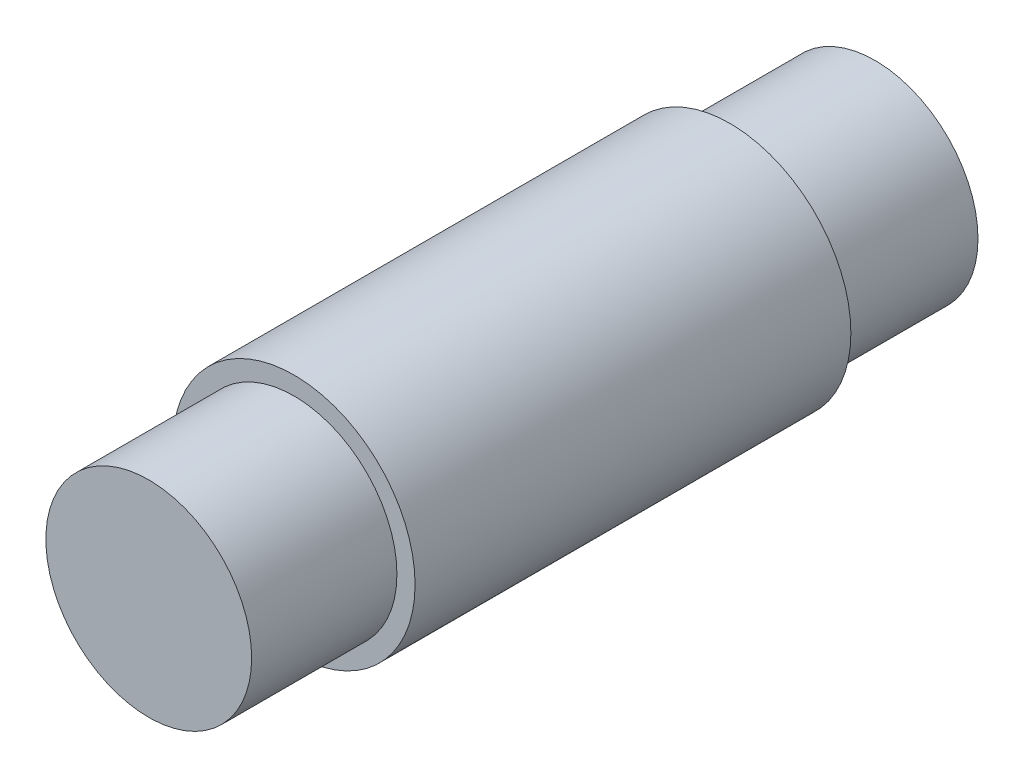
from build123d import *

# Parameters (mm, degrees)
SKETCH_1_R      = 10
EXTRUDE_1_DEPTH = 18
SKETCH_2_R      = 8.5
EXTRUDE_2_DEPTH = 12


with BuildPart() as part:
    # 草图1 → 凸台-拉伸1 (new, symmetric)
    with BuildSketch(Plane.XY):
        Circle(SKETCH_1_R)
    extrude(amount=EXTRUDE_1_DEPTH, both=True)

    # 草图2 → 凸台-拉伸2 (add)
    with BuildSketch(Plane.XY.offset(18)):
        Circle(SKETCH_2_R)
    extrude_2 = extrude(amount=EXTRUDE_2_DEPTH)

    # 镜向1: 凸台-拉伸2 across plane
    add(extrude_2.mirror(Plane.XY))


solid = part.part
